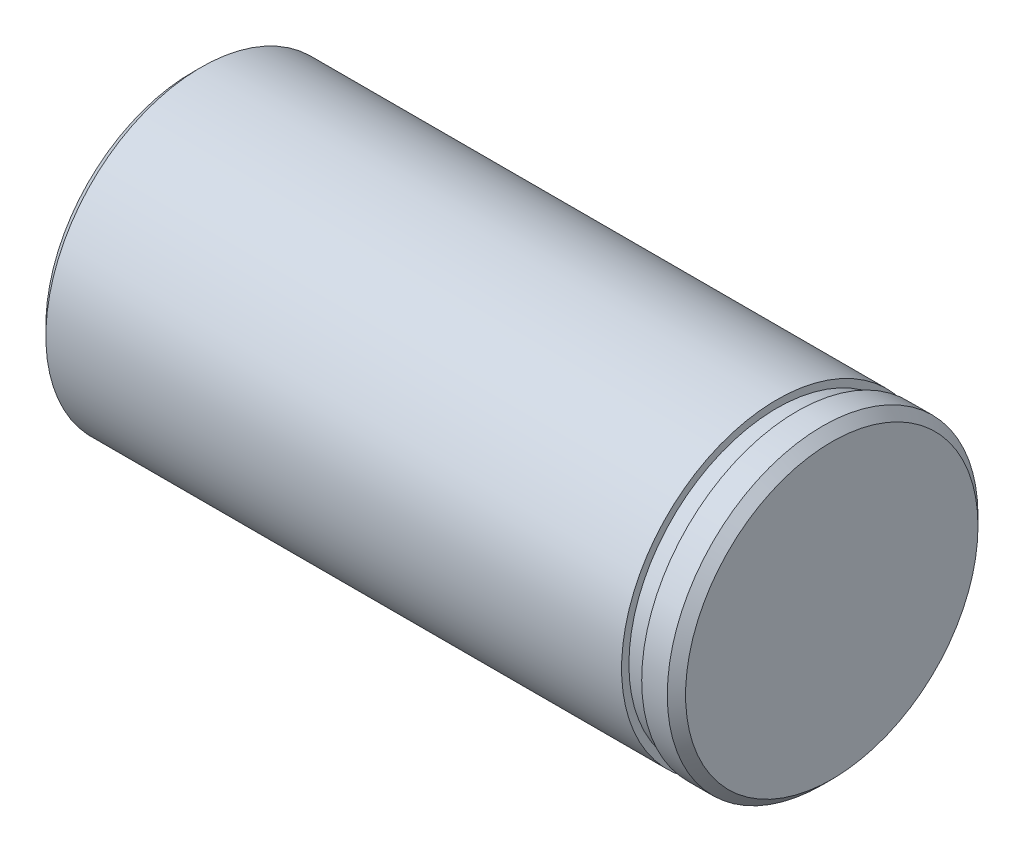
from build123d import *

# Parameters (mm, degrees)
SKETCH_1_R             = 8.5
EXTRUDE_1_DEPTH        = 35
HOLE_WIZARD_M6_1_D     = 5
HOLE_WIZARD_M6_1_DEPTH = 15
HOLE_WIZARD_M6_1_TIP   = 1.502151548
CHAMFER_1_SIZE         = 0.5
SKETCH_4_W             = 1.1
SKETCH_4_H             = 2.765489895


with BuildPart() as part:
    # 草图1 → 凸台-拉伸1 (new body)
    with BuildSketch(Plane(origin=(0, 0, 0), x_dir=(0, 0, -1), z_dir=(1, 0, 0))):
        Circle(SKETCH_1_R)
    extrude(amount=EXTRUDE_1_DEPTH)

    # M6 螺纹孔1
    with Locations(Plane.ZY):
        with Locations((0, 0)):
            Hole(HOLE_WIZARD_M6_1_D / 2, depth=HOLE_WIZARD_M6_1_DEPTH)
            with Locations((0, 0, -(HOLE_WIZARD_M6_1_DEPTH + HOLE_WIZARD_M6_1_TIP / 2))):  # 118° drill point
                Cone(0, HOLE_WIZARD_M6_1_D / 2, HOLE_WIZARD_M6_1_TIP, mode=Mode.SUBTRACT)

    # 倒角1
    chamfer_1_edges = [part.edges().sort_by_distance(p)[0] for p in [
        (0, 0, 8.5),
        (35, 0, 8.5),
    ]]
    chamfer(chamfer_1_edges, length=CHAMFER_1_SIZE)

    # 草图4 → 切除-旋转1 (revolve, cut)
    with BuildSketch(Plane(origin=(0, 0, 0), x_dir=(1, 0, 0), z_dir=(0, 1, 0)), mode=Mode.PRIVATE) as cut_revolve_1_sk:
        with Locations((32.55, 9.482744948)):
            Rectangle(SKETCH_4_W, SKETCH_4_H)
    revolve(cut_revolve_1_sk.sketch.rotate(Axis((-5.277682127, 0, 0), (1, 0, 0)), 180), axis=Axis((-5.277682127, 0, 0), (1, 0, 0)), mode=Mode.SUBTRACT)


solid = part.part
